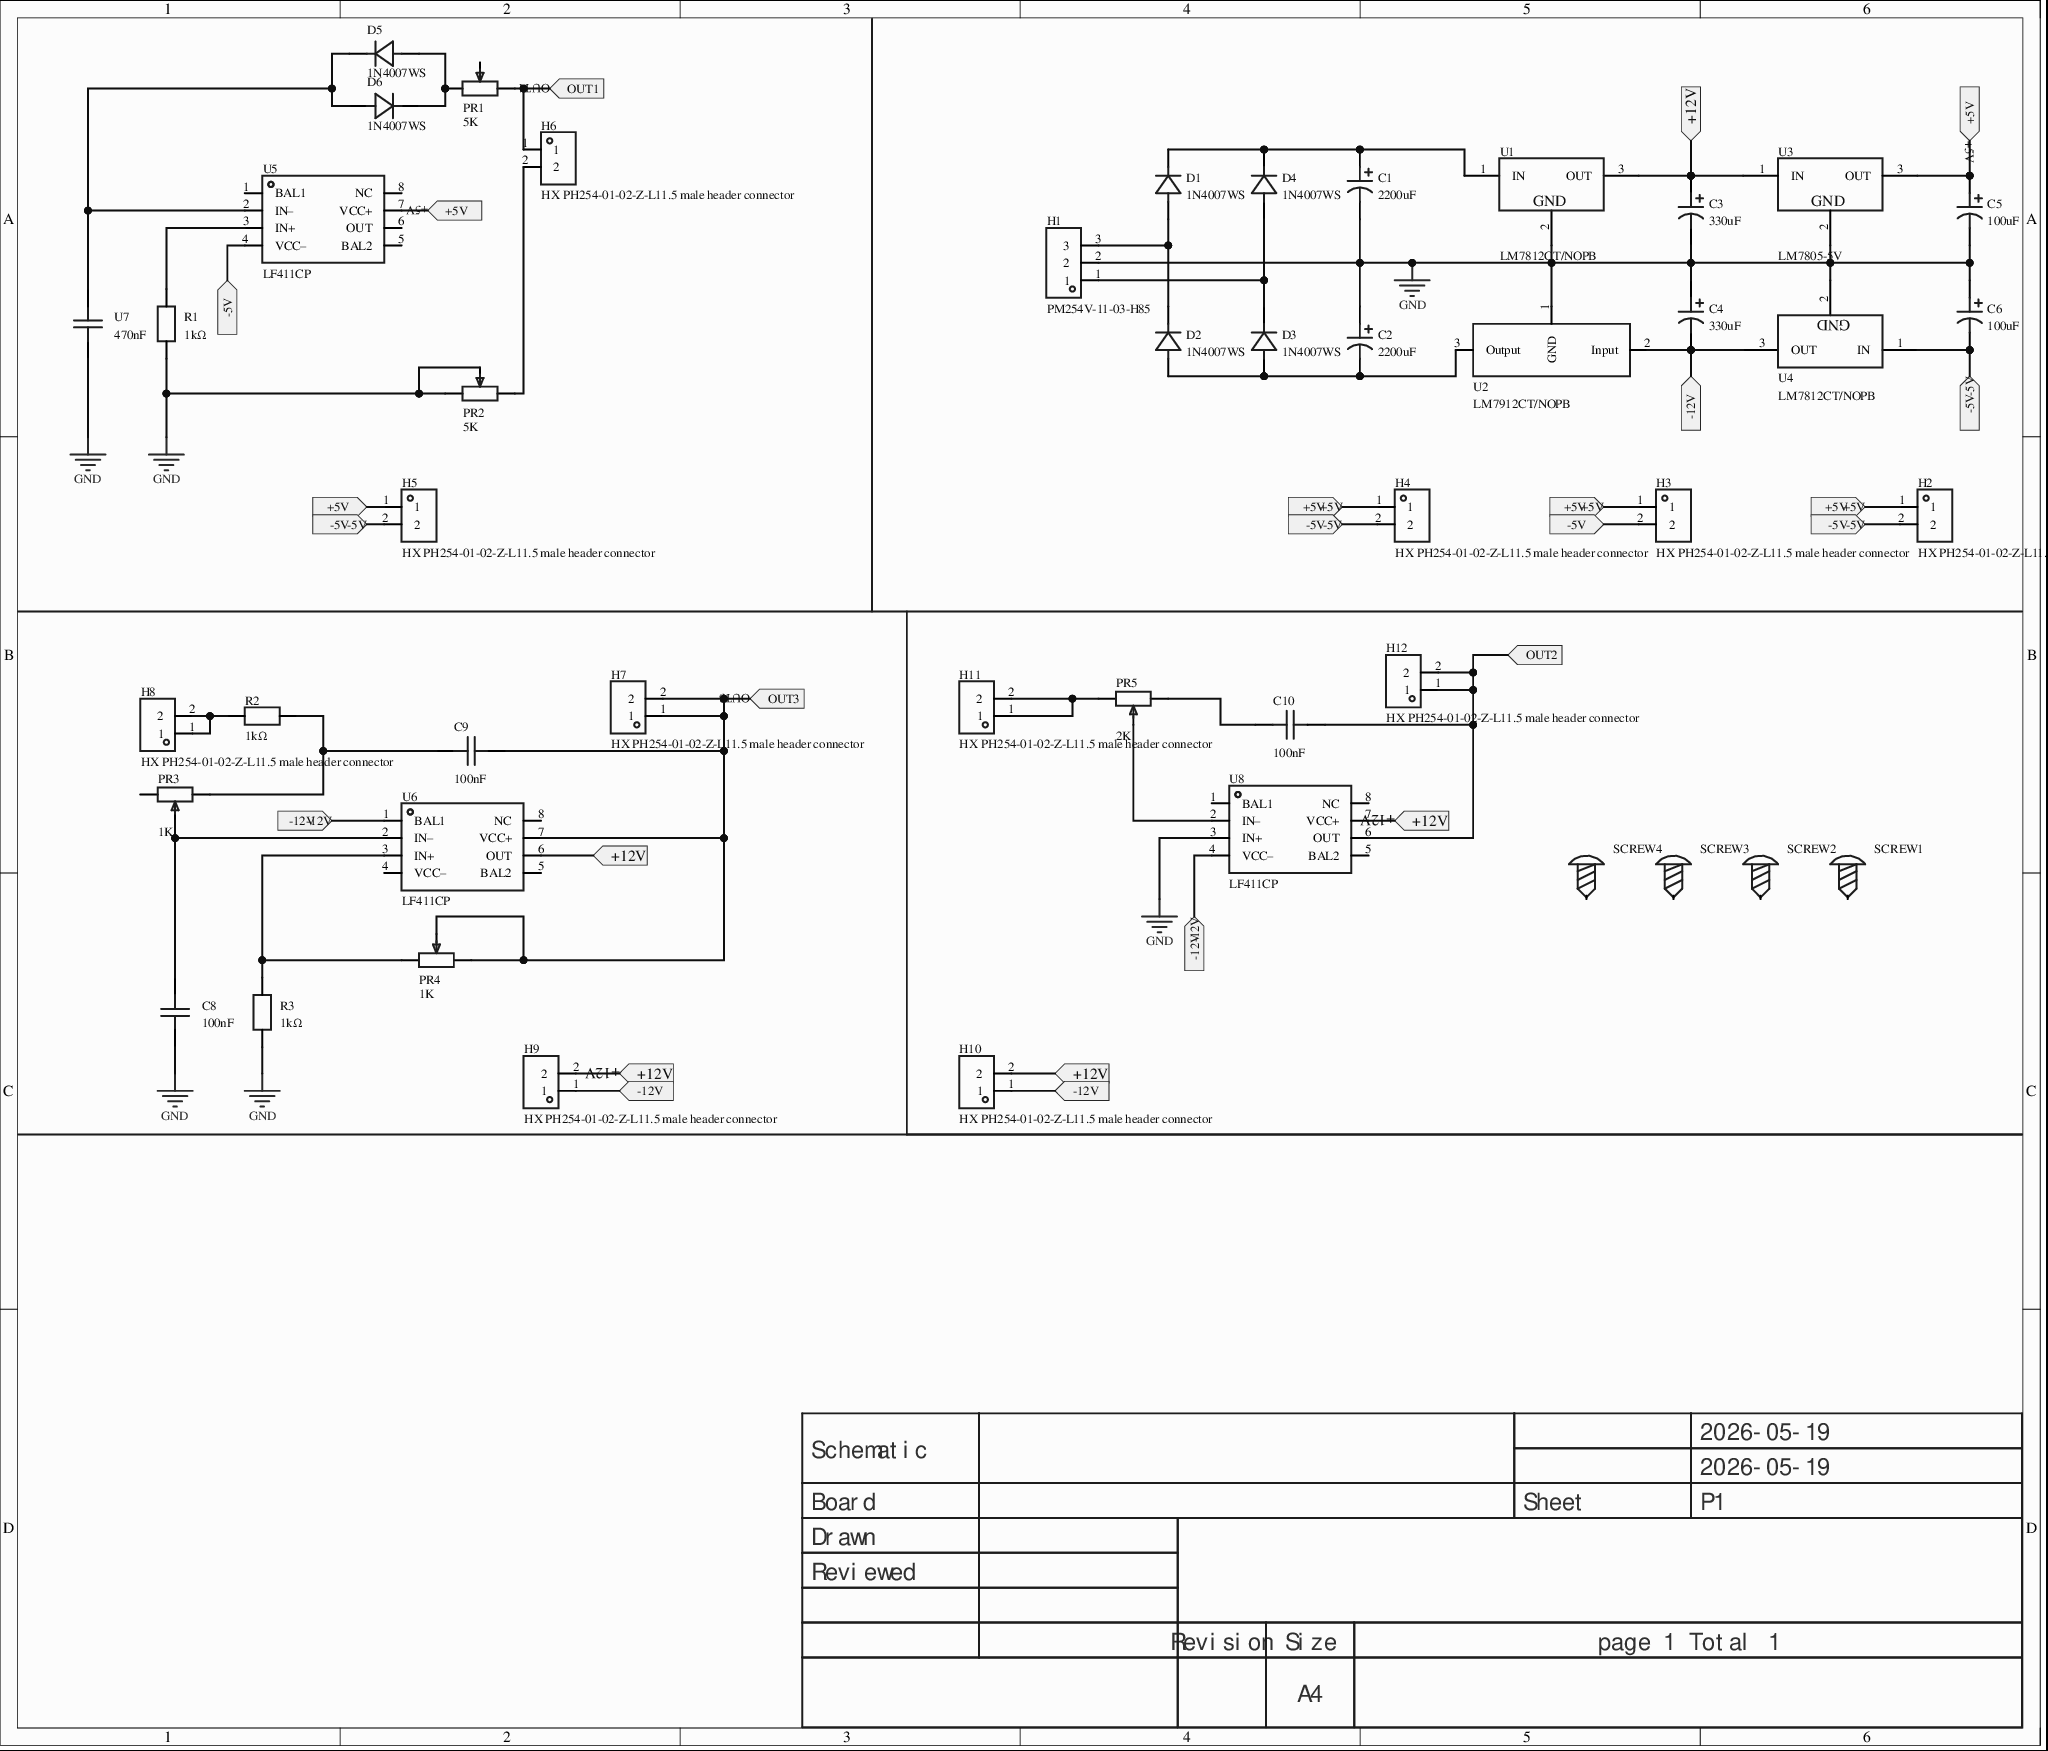
[diagram p0: MISC75076-3.schdoc]
# Altium project MISC75076-2.PrjPcb
1 sheet, 47 parts. Net scope: flat (ports and power ports of the same name join across sheets).
Board file: MISC75076.pcbdoc

## Sheet MISC75076-3.schdoc
size 297 x 254 mm; Version: V1.0; @Project Name: MISC75076; @Update Date: 2026-05-19; @Create Date: 2026-05-19; @Board Name: MISC75076; @Create Time: 19:12:04; @Page Count: 1; @Page No: 1; @Schematic Name: MISC75076; @Update Time: 19:12:04; Size: A4

### Parts
C1  2200uF  [CAP-TH_BD16.0-P7.50-D0.8-FD]
C2  2200uF  [CAP-TH_BD16.0-P7.50-D0.8-FD]
C3  330uF  [CAP-SMD_BD6.3-L6.6-W6.6-LS7.2-FD_3]
C4  330uF  [CAP-SMD_BD6.3-L6.6-W6.6-LS7.2-FD_3]
C5  100uF  [CAP-SMD_BD6.3-L6.6-W6.6-LS7.3-FD-H7.7]
C6  100uF  [CAP-SMD_BD6.3-L6.6-W6.6-LS7.3-FD-H7.7]
C8  100nF  [CAP-TH_L5.0-W2.5-P2.54-D0.7]
C9  100nF  [CAP-TH_L5.0-W2.5-P2.54-D0.7]
C10  100nF  [CAP-TH_L5.0-W2.5-P2.54-D0.7]
D1  1N4007WS  [SOD-323_L1.7-W1.3-LS2.5-RD]
D2  1N4007WS  [SOD-323_L1.7-W1.3-LS2.5-RD]
D3  1N4007WS  [SOD-323_L1.7-W1.3-LS2.5-RD]
D4  1N4007WS  [SOD-323_L1.7-W1.3-LS2.5-RD]
D5  1N4007WS  [SOD-323_L1.7-W1.3-LS2.5-RD]
D6  1N4007WS  [SOD-323_L1.7-W1.3-LS2.5-RD]
H1  PM254V-11-03-H85  [HDR-TH_3P-P2.54-V-F]
H2  HX PH254-01-02-Z-L11.5 male header connector  [HDR-TH_2P-P2.54-V-M]
H3  HX PH254-01-02-Z-L11.5 male header connector  [HDR-TH_2P-P2.54-V-M]
H4  HX PH254-01-02-Z-L11.5 male header connector  [HDR-TH_2P-P2.54-V-M]
H5  HX PH254-01-02-Z-L11.5 male header connector  [HDR-TH_2P-P2.54-V-M]
H6  HX PH254-01-02-Z-L11.5 male header connector  [HDR-TH_2P-P2.54-V-M]
H7  HX PH254-01-02-Z-L11.5 male header connector  [HDR-TH_2P-P2.54-V-M]
H8  HX PH254-01-02-Z-L11.5 male header connector  [HDR-TH_2P-P2.54-V-M]
H9  HX PH254-01-02-Z-L11.5 male header connector  [HDR-TH_2P-P2.54-V-M]
H10  HX PH254-01-02-Z-L11.5 male header connector  [HDR-TH_2P-P2.54-V-M]
H11  HX PH254-01-02-Z-L11.5 male header connector  [HDR-TH_2P-P2.54-V-M]
H12  HX PH254-01-02-Z-L11.5 male header connector  [HDR-TH_2P-P2.54-V-M]
PR1  5K  [R_3386P]
PR2  5K  [R_3386P]
PR3  1K  [R_3386P]
PR4  1K  [R_3386P]
PR5  2K  [R_3386P]
R1  1kΩ  [R0603]
R2  1kΩ  [R0603]
R3  1kΩ  [R0603]
SCREW1  (no value)  [M2螺丝]
SCREW2  (no value)  [M2螺丝]
SCREW3  (no value)  [M2螺丝]
SCREW4  (no value)  [M2螺丝]
U1  LM7812CT/NOPB  [TO-220-3_L10.2-W4.6-P2.54-L]
U2  LM7912CT/NOPB  [TO-220-3_L10.2-W4.6-P2.54-L]
U3  LM7805-5V  [TO-252-2_L6.6-W6.1-P4.58-LS9.9-TL]
U4  LM7812CT/NOPB  [TO-220-3_L10.2-W4.6-P2.54-L]
U5  LF411CP  [PDIP-8_L9.3-W6.4-P2.54-LS7.9-BL-1]
U6  LF411CP  [PDIP-8_L9.3-W6.4-P2.54-LS7.9-BL-1]
U7  470nF  [CAP-TH_L4.8-W2.4-P5.08-D0.6]
U8  LF411CP  [PDIP-8_L9.3-W6.4-P2.54-LS7.9-BL-1]

### Ports
+5V (in), +12V (in), -5V (in), -12V (in), OUT1 (in), OUT2 (in), OUT3 (in)

### Nets
GND: C1.2 C2.1 C3.2 C4.1 C5.2 C6.1 C8.2 H1.2 PR2.2 PR2.3 R1.1 R3.1 U1.2(GND) U2.1(GND) U3.2(GND) U4.2(GND) U7.1 U8.3(IN+)
+5V: C5.1 H2.1 H3.1 H4.1 H5.1 U3.3(OUT) U5.7(VCC+) ; port +5V
+12V: C3.1 H9.2 H10.2 U1.3(OUT) U3.1(IN) U6.6(OUT) U8.7(VCC+) ; port +12V
-5V: C6.2 H2.2 H3.2 H4.2 H5.2 U4.1(IN) U5.4(VCC–) ; port -5V
-12V: C4.2 H9.1 H10.1 U2.2(Input) U4.3(OUT) U6.1(BAL1) U8.4(VCC–) ; port -12V
OUT1: H6.1 PR1.1 ; port OUT1
OUT3: C9.2 H7.1 H7.2 PR4.1 PR4.2 U6.7(VCC+) ; port OUT3
NetC1_1: C1.1 D1.1(C) D4.1(C) U1.1(IN)
NetC2_2: C2.2 D2.2(A) D3.2(A) U2.3(Output)
NetC8_1: C8.1 PR3.2 U6.2(IN–)
NetC9_1: C9.1 PR3.3 R2.2
NetC10_1: C10.1 PR5.3
NetC10_2: C10.2 H12.1 H12.2 U8.6(OUT) ; port OUT2
NetD1_2: D1.2(A) D2.1(C) H1.3
NetD3_1: D3.1(C) D4.2(A) H1.1
NetD5_1: D5.1(C) D6.2(A) U5.2(IN–) U7.2
NetD5_2: D5.2(A) D6.1(C) PR1.3
NetH6_2: H6.2 PR2.1
NetH8_1: H8.1 H8.2 R2.1
NetH11_1: H11.1 H11.2 PR5.1
NetPR4_3: PR4.3 R3.2 U6.3(IN+)
NetPR5_2: PR5.2 U8.2(IN–)
NetR1_2: R1.2 U5.3(IN+)

Not connected (* = marked no-connect by the designer): PR1 2; PR3 1; SCREW1 1; SCREW2 1; SCREW3 1; SCREW4 1; U5 1(BAL1)* 5(BAL2)* 6(OUT) 8(NC)*; U6 4(VCC–)* 5(BAL2)* 8(NC)*; U8 1(BAL1)* 5(BAL2)* 8(NC)*

### Notes on the sheet
- 2026-05-19
- Schematic
- Board
- Sheet
- P1
- Drawn
- Reviewed
- Revision
- Size
- A4
- page 1 Total 1

### Library data of the parts
C1 C2 = ERA35V2200M16X26: Capacitance:2200uF;Tolerance:±20%;Rated voltage:35V;; Manufacturer: JIERR(捷而瑞); 3D Model: a842c2f395fb430083900292157136350819f05c4eef4c71ace90d822a990e87; 3D Model Transform: 629.92,629.92,0,0,0,0,0,0,-196.85; Tolerance: ±20%; Voltage Rating: 35V; Pin Spacing: 7.5mm; Lifetime: 2000hrs@105℃; AddInBom: yes; ModelName: CAP-TH_BD16.0-P7.5-D0.8-FD; Symbol: ERA35V2200M16X26; Device: ERA35V2200M16X26; LCSC Part Name: 2200uF ±20% 35V; Supplier Part: C49256808; Manufacturer Part: ERA35V2200M16X26; Supplier Footprint: 插件,D16xL26mm; JLCPCB Part Class: Extended Part; Datasheet: https://item.szlcsc.com/datasheet/ERA35V2200M16X26/51692208.html; Supplier: LCSC; Value: 2200uF; Diameter: 16mm; Height - Seated (Max): 26mm; Operating Temperature: -40℃~+105℃; ConvertToPcb: yes; FootprintName: CAP-TH_BD16.0-P7.50-D0.8-FD
C3 C4 = RVT16V330M6X8: Capacitance:330uF;Tolerance:±20%;Rated voltage:16V;Ripple current:105mA@120Hz;Equivalent series resistance (ESR):-;; Manufacturer: JIERR(捷而瑞); 3D Model: 0fb5a32acd664192a8ced5dba101c72a0819f05c4eef4c71ace90d822a990e87; 3D Model Transform: 283.464,259.842,0,0,0,0,0,0,0; Tolerance: ±20%; Voltage Rating: 16V; Lifetime: 2000hrs@105℃; AddInBom: yes; ModelName: CAP-SMD_BD6.3-L6.6-W6.6-H5.4-LS7.2-FD; Symbol: RVT16V330M6X8; Device: RVT16V330M6X8; LCSC Part Name: 330uF ±20% 16V; Supplier Part: C47023104; Manufacturer Part: RVT16V330M6X8; Supplier Footprint: SMD,D6.3xL7.7mm; JLCPCB Part Class: Extended Part; Datasheet: https://item.szlcsc.com/datasheet/RVT16V330M6X8/49206205.html; Supplier: LCSC; Value: 330uF; Ripple Current: 105mA@120Hz; Equivalent Series Resistance(ESR): -; Diameter: 6.3mm; Height - Seated (Max): 7.7mm; Operating Temperature: -40℃~+105℃; ConvertToPcb: yes; FootprintName: CAP-SMD_BD6.3-L6.6-W6.6-LS7.2-FD_3
C5 C6 = JVJ50V100M6x8: Capacitance:100uF;Tolerance:±20%;Rated voltage:50V;Ripple current:140mA@120Hz;; Manufacturer: JIERR(捷而瑞); 3D Model: ccbda52dceed4b139172c40f75c9da3f0819f05c4eef4c71ace90d822a990e87; 3D Model Transform: 287.401,259.842,0,0,0,0,0,0,0; Tolerance: ±20%; Voltage Rating: 50V; Lifetime: 2000hrs@105℃; AddInBom: yes; Symbol: JVJ50V100M6X8; Device: JVJ50V100M6x8; LCSC Part Name: 100uF ±20% 50V; Supplier Part: C46550415; Manufacturer Part: JVJ50V100M6x8; Supplier Footprint: SMD,D6.3xL7.7mm; JLCPCB Part Class: Extended Part; Datasheet: https://item.szlcsc.com/datasheet/JVJ50V100M6x8/48680109.html; Supplier: LCSC; Value: 100uF; Ripple Current: 140mA@120Hz; Diameter: 6.3mm; Height - Seated (Max): 7.7mm; Operating Temperature: -55℃~+105℃; ConvertToPcb: yes; FootprintName: CAP-SMD_BD6.3-L6.6-W6.6-LS7.3-FD-H7.7; ModelName: CAP-SMD_BD6.3-L6.6-W6.6-LS7.3-FD-H7.7
C8-C10 = CC1H104ZA1PD3F5P3003: Capacitance:100nF;Tolerance:-20%~+80%;Rated voltage:50V;Temperature coefficient:Y5V;; Manufacturer: Dersonic(德尔创); 3D Model: ad23374a1d7d4d08a9199c602c7613e00819f05c4eef4c71ace90d822a990e87; 3D Model Transform: 196.785,98.425,0,0,0,0,0,0,-137.795; Voltage Rating: 50V; Pin Spacing: 2.54mm; Temperature Coefficient: Y5V; Body Thickness: 2.4mm; AddInBom: yes; ModelName: CAP-TH_BD5.0-W2.5-P2.54; Symbol: CC1H104ZA1PD3F5P3003; Device: CC1H104ZA1PD3F5P3003; LCSC Part Name: 100nF -20%~+80% 50V; Supplier Part: C353903; Manufacturer Part: CC1H104ZA1PD3F5P3003; Supplier Footprint: 插件,P=2.54mm; JLCPCB Part Class: Extended Part; Datasheet: https://item.szlcsc.com/datasheet/CC1H104ZA1PD3F5P3003/329871.html; Supplier: LCSC; Value: 100nF; Tolerance: -20%~+80%; Diameter: 5.8mm; ConvertToPcb: yes; FootprintName: CAP-TH_L5.0-W2.5-P2.54-D0.7
D1-D6 = 1N4007WS_C53055759: Diode configuration:1 single unit;Forward voltage (Vf):1.1V@1A;DC reverse voltage (Vr):1kV;Rectified current:1A;; Manufacturer: R+O(宏嘉诚); 3D Model: 0f2f330c645944df9245ac3c3fec34560819f05c4eef4c71ace90d822a990e87; 3D Model Transform: 98.425,49.2125,0,0,0,0,0,0,0; Voltage - DC Reverse(Vr): 1kV; Current - Rectified: 1A; Reverse Leakage Current (Ir): 5uA@1000V; AddInBom: yes; ModelName: SOD-323_L1.7-W1.3-LS2.5-FD; Symbol: 1N4007WS_C53055759; Device: 1N4007WS_C53055759; LCSC Part Name: 1N4007WS; Supplier Part: C53055759; Manufacturer Part: 1N4007WS; Supplier Footprint: SOD-323; JLCPCB Part Class: Extended Part; Datasheet: https://item.szlcsc.com/datasheet/1N4007WS/56000076.html; Supplier: LCSC; Diode Configuration: 1 single unit; Voltage - Forward(Vf@If): 1.1V@1A; ConvertToPcb: yes; FootprintName: SOD-323_L1.7-W1.3-LS2.5-RD
H1 = PM254V-11-03-H85: Socket structure:1x3P;Pitch:2.54mm;Row spacing:-;Round/square hole:Square hole;Mounting:Through-hole;Rows:Single row;Total holes:3P;Rated current:3A;Socket direction:Top;Plastic height:8.5mm;Contact material:Brass;Contact plating:-;Operating temperature:-40℃~+105℃;; Manufacturer: XFCN(兴飞); AddInBom: yes; ModelId: f3b3cc5aae9641bf9e56fc160cef875b0819f05c4eef4c71ace90d822a990e87; ModelName: HDR2.54-F-LI-1X3P; ModelTransform: 299.9994,100,0,0,0,0,0,0,-118.11; Holes Structure: 1x3P; Pitch: 2.54mm; Number of Positions: 3P; Current Rating: 3A; Holes Direction: Top; Symbol: PM254V-11-03-H85; Device: PM254V-11-03-H85; LCSC Part Name: 1x3P 间距:2.54mm 直插; SupplierPart: C541850; ManufacturerPart: PM254V-11-03-H85; Supplier Footprint: 插件,P=2.54mm; JLCPCB Part Class: Extended Part; Datasheet: https://item.szlcsc.com/datasheet/PM254V-11-03-H85/562471.html; Supplier: LCSC; ConvertToPcb: yes; FootprintName: HDR-TH_3P-P2.54-V-F; Row Spacing: -; Circular Hole / Square Hole: Square hole; Mounting Type: Through-hole; Number of Rows: Single row; Insulation Height: 8.5mm; Contact Material: Brass; Contact Plating: -; Operating Temperature: -40℃~+105℃
H2-H12 = HX PH254-01-02-Z-L11.5 male header connector: Pin structure:1x2P;Pitch:2.54mm;Round/square pin:Square pin;Mounting:Through-hole;Rows:Single row;Total pins:2P;Rated current:3A;Rated voltage:1kV;Mating pin length:6mm;Plastic height:2.5mm;Termination pin length:3mm;Contact material:Brass;Contact plating:Gold;Operating temperature:-40℃~+105℃;; Manufacturer: hanxia(韩下); AddInBom: yes; ModelId: e35305ec3aa84b66b849f914b715e73f0819f05c4eef4c71ace90d822a990e87; ModelName: HDR2.54-M-LI-1X2P; ModelTransform: 200,100,0,0,0,0,0,0,-118.11; Pin Structure: 1x2P; Pitch: 2.54mm; Current Rating: 3A; Voltage Rating (Max): 1kV; Symbol: HX PH254-01-02-Z-L11.5 MALE HEADER CONNECTOR; Device: HX PH254-01-02-Z-L11.5 male header connector; LCSC Part Name: 1x2P 间距:2.54mm 方针 直插; SupplierPart: C52016390; ManufacturerPart: HX PH254-01-02-Z-L11.5 male header connector; Supplier Footprint: 插件,P=2.54mm; JLCPCB Part Class: Extended Part; Datasheet: https://item.szlcsc.com/datasheet/HX%2520PH254-01-02-Z-L11.5%2520male%2520header%2520connector/54760435.html; Supplier: LCSC; ConvertToPcb: yes; FootprintName: HDR-TH_2P-P2.54-V-M; Circluar Pins/Square Pins: Square pin; Mounting Type: Through-hole; Number of Rows: Single row; Number of Pins: 2P; Length of Mating Pin: 6mm; Insulation Height: 2.5mm; Length of End Connection Pin: 3mm; Contact Material: Brass; Contact Plating: Gold; Operating Temperature: -40℃~+105℃
PR1-PR5 = R_3386P: Symbol: 3386P-1-103LF; ConvertToPcb: yes; ModelId: 6a25d8a4450b4318959c1cd98efa6b0c0819f05c4eef4c71ace90d822a990e87; ModelName: RES-ADJ-TH_3P-L9.5-W9.5-P2.54-BR-BS; ModelTransform: 375.19,375.19,387,-90,0,0,0,0,-197; Device: R_3386P; AddInBom: yes; FootprintName: R_3386P; Supplier Footprint: 直插
  PR1 PR2: Value: 5K
  PR3 PR4: Value: 1K
  PR5: Value: 2K
R1-R3 = FRH0603B1001TS: Resistor type:Thick film resistor;Resistance:1kΩ;Tolerance:±0.1%;Power:100mW;Working voltage:75V;Temperature coefficient:±100ppm/℃;; Manufacturer: FOJAN(富捷); 3D Model: fc143cca1e79419f9cd78b61e9279f080819f05c4eef4c71ace90d822a990e87; 3D Model Transform: 31.8897,63.7794,0,90,0,0,0,0,0; Tolerance: ±0.1%; Power(Watts): 100mW; Voltage-Supply(Max): 75V; AddInBom: yes; Symbol: FRH0603B1001TS; Device: FRH0603B1001TS; LCSC Part Name: 厚膜电阻 0603 1KΩ ±0.1% 100mW; Supplier Part: C49196685; Manufacturer Part: FRH0603B1001TS; Supplier Footprint: 0603; JLCPCB Part Class: Extended Part; Datasheet: https://item.szlcsc.com/datasheet/FRH0603B1001TS/51598983.html; Supplier: LCSC; Type: Thick film resistor; Value: 1kΩ; Temperature Coefficient: ±100ppm/℃; Operating Temperature: -55℃~+155℃; ConvertToPcb: yes; FootprintName: R0603; ModelName: R0603
SCREW1-SCREW4 = M2螺丝: Symbol: Screw hole; Device: M2 screw; ConvertToPcb: yes; AddInBom: yes; Supplier Footprint: 插件; FootprintName: M2 screw
U1 U4 = LM7812CT/NOPB: Output type:Fixed;Max input voltage:-;Output voltage:12V;Output current:1.5A;Power supply rejection ratio (PSRR):72dB@(120Hz);Output polarity:Positive;; Manufacturer: TI(德州仪器); AddInBom: yes; ModelId: 6197bb0aad96481ab8a17aa6d23d90f10819f05c4eef4c71ace90d822a990e87; ModelTransform: 399.999,177.204,0,0,0,0,0,24.606,-196.85; Output Type: Fixed; Output Voltage: 12V; Output Current: 1.5A; Number of Outputs: 1; Symbol: LM7812CT/NOPB; Device: LM7812CT/NOPB; LCSC Part Name: 1.5A、30V 线性稳压器; SupplierPart: C2872599; ManufacturerPart: LM7812CT/NOPB; Supplier Footprint: TO-220-3; JLCPCB Part Class: Extended Part; Datasheet: https://www.ti.com/cn/lit/gpn/lm7800; Supplier: LCSC; ConvertToPcb: yes; FootprintName: TO-220-3_L10.2-W4.6-P2.54-L; ModelName: TO-220-3_L10.2-W4.6-P2.54-L; Maximum Input Voltage: -; Power Supply Rejection Ratio (PSRR): 72dB@(120Hz); Feature: Anti-static protection; short-circuit protection; thermal shutdown (TSD); overcurrent protection (OCP); with enable; Operating Temperature: 0℃~+125℃@(Tj); Output Polarity: Positive
U2 = LM7912CT/NOPB: Output type:Fixed;Max input voltage:35V;Output voltage:12V;Output current:1.5A;Power supply rejection ratio (PSRR):70dB@(120Hz);Output polarity:Negative;; Manufacturer: TI(德州仪器); AddInBom: yes; ModelId: 6197bb0aad96481ab8a17aa6d23d90f10819f05c4eef4c71ace90d822a990e87; ModelTransform: 399.999,177.204,0,0,0,0,0,24.606,-196.85; Output Type: Fixed; Maximum Input Voltage: 35V; Output Voltage: 12V; Output Current: 1.5A; Dropout Voltage: 1.1V@(1A); standby current: 1.5mA; Number of Outputs: 1; Symbol: LM7912CT/NOPB; Device: LM7912CT/NOPB; LCSC Part Name: 1.5A 负电压线性稳压器; SupplierPart: C10116; ManufacturerPart: LM7912CT/NOPB; Supplier Footprint: TO-220-3; JLCPCB Part Class: Extended Part; Datasheet: https://www.ti.com/cn/lit/gpn/lm79; Supplier: LCSC; ConvertToPcb: yes; FootprintName: TO-220-3_L10.2-W4.6-P2.54-L; ModelName: TO-220-3_L10.2-W4.6-P2.54-L; Power Supply Rejection Ratio (PSRR): 70dB@(120Hz); Feature: Anti-static protection; thermal shutdown (TSD); overcurrent protection (OCP); Operating Temperature: 0℃~+125℃; Output Polarity: Negative
U3 = LM7805-5V_C9900008050: AddInBom: yes; ModelId: ce57f84d66384067af8a68020b6de06d0819f05c4eef4c71ace90d822a990e87; ModelName: TO-252-2L-3P_L6.6-W6.1-H2.3-LS10.1-P4.6; ModelTransform: 259.842,390.52442,0,270,0,0,39.372,0.002,0; Symbol: LM7805-5V_C9900008050; Device: LM7805-5V_C9900008050; LCSC Part Name: LM7805-5V; SupplierPart: C9900008050; ManufacturerPart: LM7805-5V; Supplier Footprint: TO-252-2; JLCPCB Part Class: Extended Part; Supplier: LCSC; ConvertToPcb: yes; FootprintName: TO-252-2_L6.6-W6.1-P4.58-LS9.9-TL
U5 U6 U8 = LF411CP: Gain-bandwidth product (GBP):3MHz;Input bias current (Ib):50pA;Input offset voltage (Vos):800uV;Slew rate (SR):13V/us;; Manufacturer: TI(德州仪器); AddInBom: yes; ModelId: 28221afe73f64733a5f69edf09cc82000819f05c4eef4c71ace90d822a990e87; ModelTransform: 366.141,322.834,0,0,0,0,0,0,-118.11; Gain Bandwidth Product(GBP): 3MHz; Current - Input Bias(Ib): 50pA; Voltage - Input Offset(Vos): 800uV; Slew Rate(SR): 13V/us; Symbol: LF411CP; Device: LF411CP; LCSC Part Name: LF411CP; SupplierPart: C1346062; ManufacturerPart: LF411CP; Supplier Footprint: PDIP-8; JLCPCB Part Class: Extended Part; Datasheet: https://www.ti.com/cn/lit/gpn/lf411; Supplier: LCSC; ConvertToPcb: yes; FootprintName: PDIP-8_L9.3-W6.4-P2.54-LS7.9-BL-1; ModelName: PDIP-8_L9.3-W6.4-P2.54-LS7.9-BL-1; Operating Temperature: 0℃~+70℃
U7 = 178MU0009: Capacitance:470nF;Tolerance:±10%;Rated voltage:50V;Temperature coefficient:X7R;; Manufacturer: KNSCHA(科尼盛); 3D Model: 723c35d9c0ee4f1b9d74cee04ca966cb0819f05c4eef4c71ace90d822a990e87; 3D Model Transform: 231.496,95.01753,0,0,0,0,0,0,-196.85; Tolerance: ±10%; Voltage Rating: 50V; Temperature Coefficient: X7R; Pin Spacing: 5.08mm; AddInBom: yes; Symbol: 178MU0009; Device: 178MU0009; LCSC Part Name: 470nF ±10% 50V; Supplier Part: C5632433; Manufacturer Part: 178MU0009; Supplier Footprint: 插件,P=5.08mm; JLCPCB Part Class: Extended Part; Datasheet: https://item.szlcsc.com/datasheet/178MU0009/6552588.html; Supplier: LCSC; Value: 470nF; ConvertToPcb: yes; FootprintName: CAP-TH_L4.8-W2.4-P5.08-D0.6; ModelName: CAP-TH_L4.8-W2.4-P5.08-D0.6